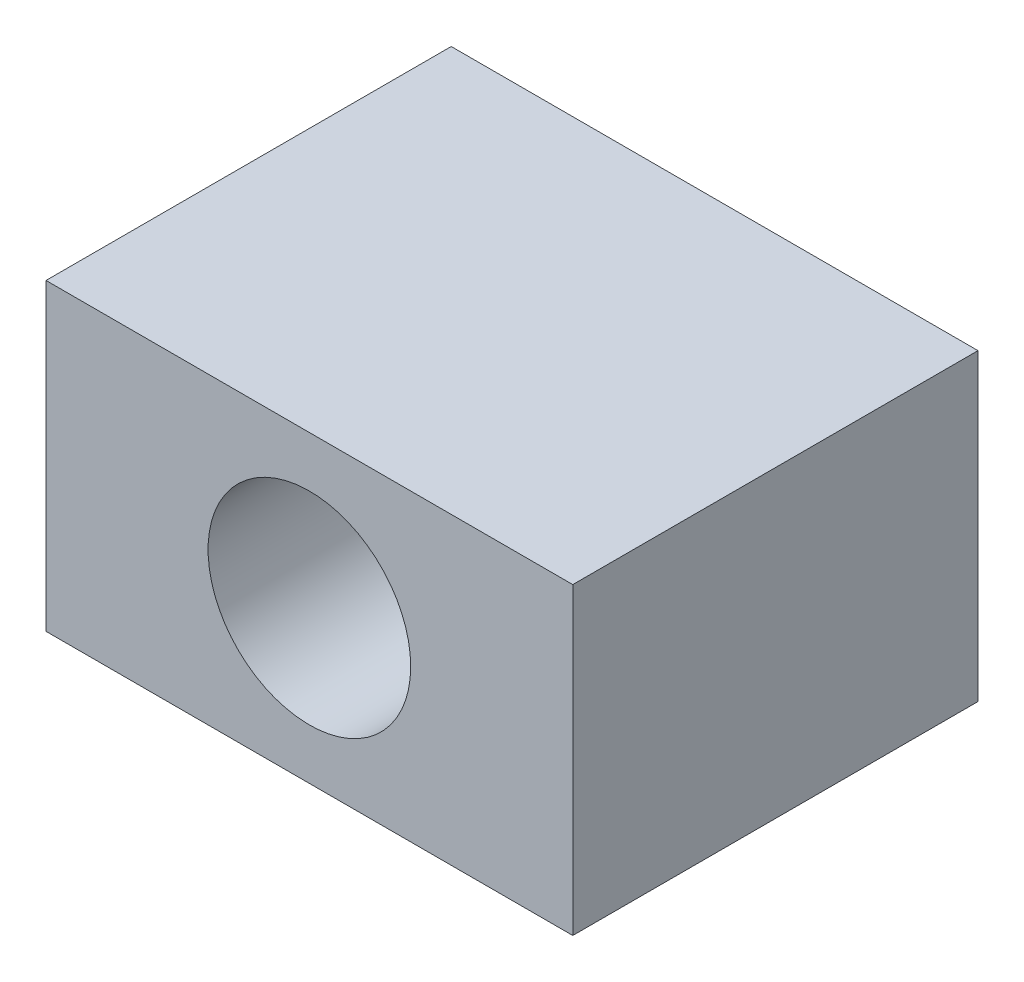
SolidWorks part; units mm, degrees
ref_plane "Front Plane" through (0, 0, 0) normal (0, 0, 1) x (1, 0, 0)
ref_plane "Top Plane" through (0, 0, 0) normal (0, 1, 0) x (1, 0, 0)
ref_plane "Right Plane" through (0, 0, 0) normal (1, 0, 0) x (0, 0, -1)
sketch "Sketch1" plane through (0, 0, 0) normal (0, 0, 1) x (1, 0, 0)
  line L1 (-13, 7.5) -> (13, 7.5)
  line L2 (-13, 7.5) -> (-13, -7.5)
  line L3 (-13, -7.5) -> (13, -7.5)
  line L4 (13, 7.5) -> (13, -7.5)
  line L5 (-13, 7.5) -> (13, -7.5) construction
  line L6 (-13, -7.5) -> (13, 7.5) construction
  circle A0 centre (0, 0) radius 5
  point P0 (0, 0)
  dimension "D3" = 10
  dimension "D1" = 26
  dimension "D2" = 15
extrude "Boss-Extrude1" add sketch "Sketch1" along normal blind 20
